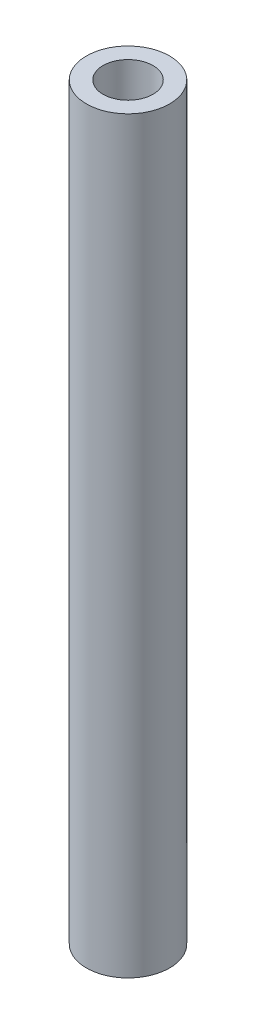
SolidWorks part; units mm, degrees
ref_plane "Front Plane" through (0, 0, 0) normal (0, 0, 1) x (1, 0, 0)
ref_plane "Top Plane" through (0, 0, 0) normal (0, 1, 0) x (1, 0, 0)
ref_plane "Right Plane" through (0, 0, 0) normal (1, 0, 0) x (0, 0, -1)
sketch "Sketch1" plane through (0, 0, 0) normal (0, 1, 0) x (1, 0, 0)
  circle A0 centre (0, 0) radius 2.5
  circle A1 centre (0, 0) radius 1.5
  dimension "D1" = 5
  dimension "D2" = 3
extrude "Boss-Extrude1" add sketch "Sketch1" along normal blind 45
cosmetic thread "Cosmetic Thread1" parameters "D1"=5, "D2"=4
sketch "Sketch2" plane through (0, 0, 0) normal (0, -1, 0) x (1, 0, 0)
  circle A0 centre (0, 0) radius 1.5 construction
  circle A1 centre (0, 0) radius 1.5
  circle A2 centre (0, 0) radius 0.5
  dimension "D1" = 1
extrude "Boss-Extrude2" add sketch "Sketch2" against normal blind 2
